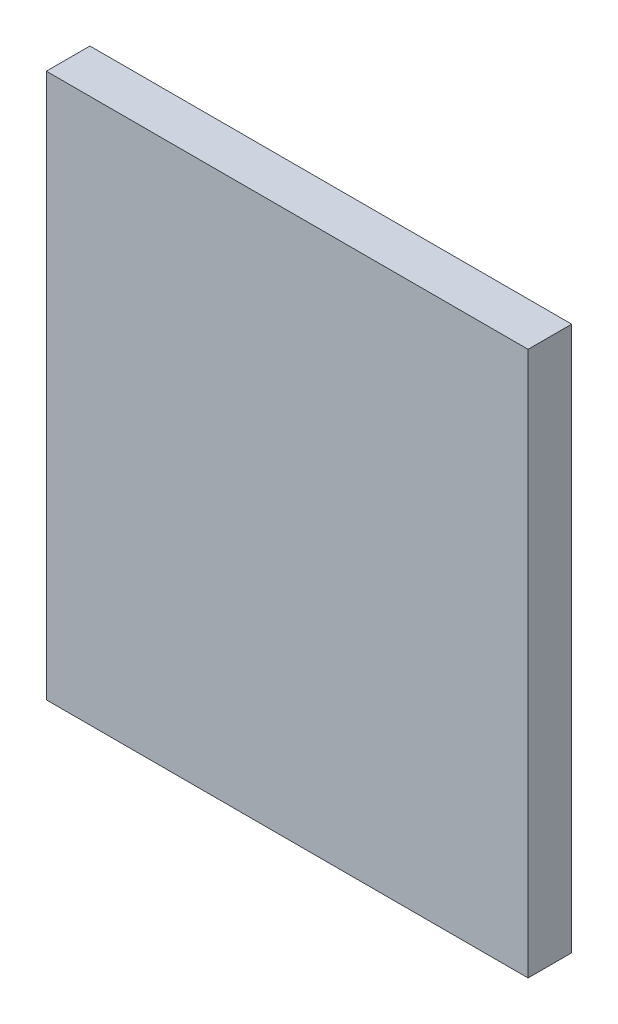
from build123d import *

# Parameters (mm, degrees)
SKETCH1_W           = 110.487143692
SKETCH1_H           = 124.867894346
BOSS_EXTRUDE1_DEPTH = 10


with BuildPart() as part:
    # Sketch1 → Boss-Extrude1 (new body)
    with BuildSketch(Plane.XY):
        with Locations((-0.740380611, 1.355088617)):
            Rectangle(SKETCH1_W, SKETCH1_H)
    extrude(amount=BOSS_EXTRUDE1_DEPTH)


solid = part.part
